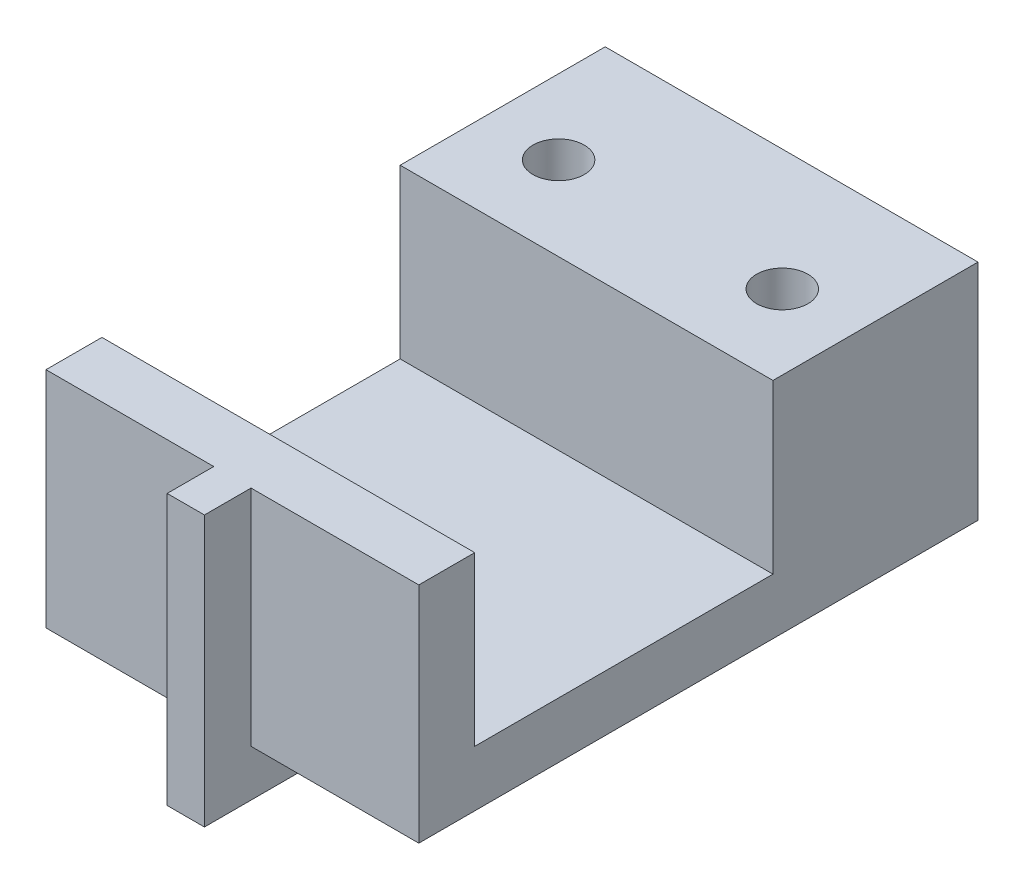
from build123d import *

# Parameters (mm, degrees)
SKETCH1_W                                    = 40
SKETCH1_H                                    = 60
BOSS_EXTRUDE1_DEPTH                          = 24
SKETCH4_W                                    = 38
SKETCH4_H                                    = 18
CUT_EXTRUDE2_DEPTH                           = 83
SKETCH5_W                                    = 4
SKETCH5_H                                    = 60
BOSS_EXTRUDE2_DEPTH                          = 5
SKETCH6_W                                    = 4
SKETCH6_H                                    = 11
BOSS_EXTRUDE3_DEPTH                          = 5
SKETCH7_W                                    = 40
SKETCH7_H                                    = 6
BOSS_EXTRUDE4_DEPTH                          = 18
CBORE_FOR_M5_HEXAGON_SOCKET_HEAD_CAP_2_COUNT = 2
CBORE_FOR_M5_HEXAGON_SOCKET_HEAD_CAP_2_PITCH = 24
SKETCH11_W                                   = 4
SKETCH11_H                                   = 5
BOSS_EXTRUDE5_DEPTH                          = 18


with BuildPart() as part:
    # Sketch1 → Boss-Extrude1 (new body)
    with BuildSketch(Plane(origin=(0, 0, 0), x_dir=(1, 0, 0), z_dir=(0, 1, 0))):
        Rectangle(SKETCH1_W, SKETCH1_H)
    extrude(amount=BOSS_EXTRUDE1_DEPTH)

    # Sketch4 → Cut-Extrude2 (cut)
    with BuildSketch(Plane.ZY.offset(20)):
        with Locations((11, 15)):
            Rectangle(SKETCH4_W, SKETCH4_H)
    extrude(amount=-CUT_EXTRUDE2_DEPTH, mode=Mode.SUBTRACT)

    # Sketch5 → Boss-Extrude2 (add)
    with BuildSketch(Plane.XZ):
        Rectangle(SKETCH5_W, SKETCH5_H)
    extrude(amount=BOSS_EXTRUDE2_DEPTH)

    # Sketch6 → Boss-Extrude3 (add)
    with BuildSketch(Plane.XY.offset(30)):
        with Locations((0, 0.5)):
            Rectangle(SKETCH6_W, SKETCH6_H)
    extrude(amount=BOSS_EXTRUDE3_DEPTH)

    # Sketch7 → Boss-Extrude4 (add)
    with BuildSketch(Plane(origin=(0, 6, 0), x_dir=(1, 0, 0), z_dir=(0, 1, 0))):
        with Locations((0, -27)):
            Rectangle(SKETCH7_W, SKETCH7_H)
    extrude(amount=BOSS_EXTRUDE4_DEPTH)

    # Sketch10 → CBORE for M5 Hexagon socket head cap screws1 (revolve, cut)
    with BuildSketch(Plane(origin=(12, 0, -17), x_dir=(0, 0, -1), z_dir=(1, 0, 0))):
        Polygon((0, 0), (0, 24), (2.75, 24), (2.75, 5.7), (5, 5.7), (5, 0.025), (5.025, 0), align=None)
    cbore_for_m5_hexagon_socket_head_cap_scr = revolve(axis=Axis((12, -6.35, -17), (0, 1, 0)), mode=Mode.SUBTRACT)

    # CBORE for M5 Hexagon socket head cap 2: CBORE for M5 Hexagon socket head cap screws1 ×2
    with Locations(*[(-i * CBORE_FOR_M5_HEXAGON_SOCKET_HEAD_CAP_2_PITCH, 0, 0) for i in range(1, CBORE_FOR_M5_HEXAGON_SOCKET_HEAD_CAP_2_COUNT)]):
        add(cbore_for_m5_hexagon_socket_head_cap_scr, mode=Mode.SUBTRACT)

    # Sketch11 → Boss-Extrude5 (add)
    with BuildSketch(Plane(origin=(0, 6, 0), x_dir=(1, 0, 0), z_dir=(0, 1, 0))):
        with Locations((0, -32.5)):
            Rectangle(SKETCH11_W, SKETCH11_H)
    extrude(amount=BOSS_EXTRUDE5_DEPTH)


solid = part.part
